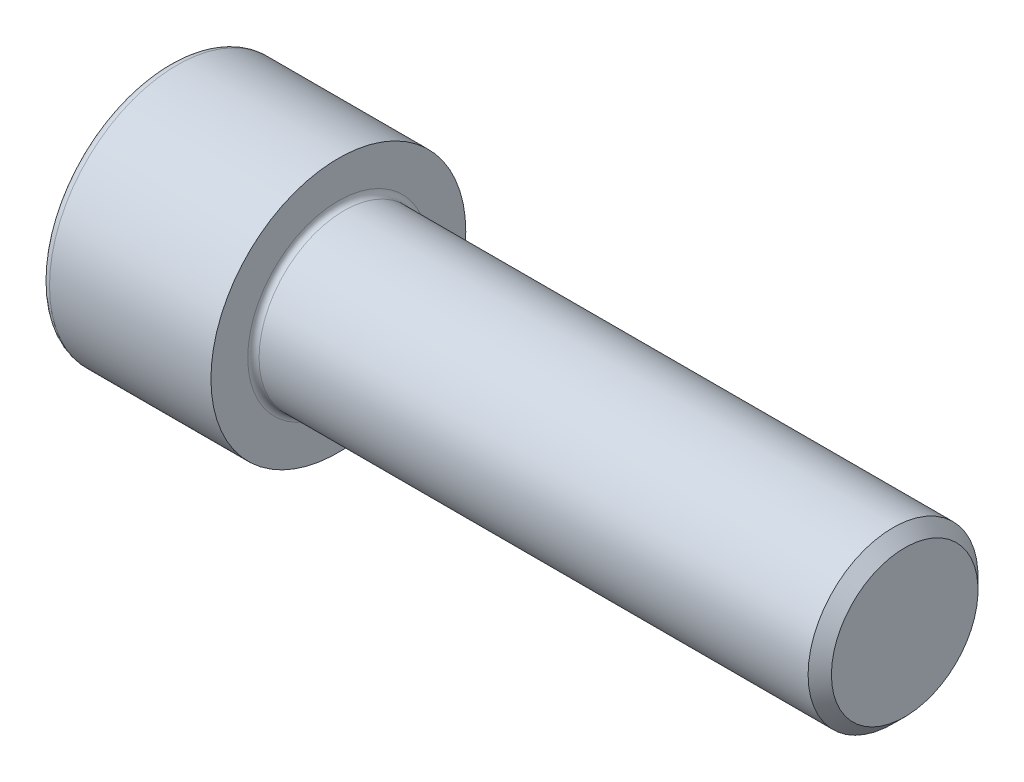
SolidWorks part; units mm, degrees
revolve "Base-Revolve" add sketch "BodySke"
sketch "BodySke" plane through (0, 0, 0) normal (0, 0, 1) x (1, 0, 0)
  line L0 (0, 0) -> (0, 18)
  line L1 (0, 18) -> (24, 18)
  line L2 (24, 18) -> (24, 12)
  line L3 (24, 12) -> (102.352, 12)
  line L4 (104, 10.352) -> (104, 0)
  line L5 (104, 0) -> (0, 0)
  line L6 (-31.75, 0) -> (127, 0) construction
  line L8 (104, 10.352) -> (102.352, 12)
  line L10 (104, -10.352) -> (102.352, -12) construction
  line L11 (27, 9.525) -> (27, 3.175) construction
  line L12 (44, 9.525) -> (44, 3.175) construction
  line L13 (44, 9.525) -> (44, 3.175) construction
cosmetic thread "ThreadCosmetic" [suppressed]
fillet "Fillet1" radius 0.8 1 edges at (24, 0, 12)
fillet "Fillet2" radius 1.2 1 edges at (0, 0, 18)
ref_plane "Plane1" through (0, 0, 0) normal (0, 0, 1) x (1, 0, 0)
ref_plane "Plane2" through (0, 0, 0) normal (0, 1, 0) x (1, 0, 0)
ref_plane "Plane3" through (0, 0, 0) normal (1, 0, 0) x (0, 0, -1)
other "Configuration Table"
sketch "Sketch2" plane through (0, 0, 0) normal (0, 0, 1) x (1, 0, 0)
  line L0 (0, 9.6375) -> (12.573, 9.6375)
  line L1 (12.573, 9.6375) -> (18.1372, 0)
  line L2 (-31.75, 0) -> (127, 0) construction
  line L3 (18.1372, 0) -> (0, 0)
  line L4 (0, 0) -> (0, 9.6375)
  line L6 (0, 0) -> (47.625, 0) construction
revolve "Hex-PreBroach" cut sketch "Sketch2" angle 360 about L6
sketch "Sketch3" plane through (0, 0, 0) normal (-1, 0, 0) x (0, 0.5, 0.866)
  line L0 (5.5642, 9.6375) -> (-5.5642, 9.6375)
  line L1 (-5.5642, 9.6375) -> (-11.1284, 0)
  line L2 (5.5642, 9.6375) -> (11.1284, 0)
  line L3 (5.5642, -9.6375) -> (11.1284, 0)
  line L4 (5.5642, -9.6375) -> (-5.5642, -9.6375)
  line L5 (-5.5642, -9.6375) -> (-11.1284, 0)
extrude "Hex" cut sketch "Sketch3" against normal blind 12.573
sketch "ThdSchSke" plane through (0, 0, 0) normal (0, 0, 1) x (1, 0, 0)
  line L0 (44, -10.352) -> (42.8461, -12)
  line L1 (44, -10.352) -> (45.1539, -12)
  line L2 (45.1539, -12) -> (45.1539, -15)
  line L3 (-3.175, 0) -> (5.1513, 0) construction
  line L4 (0, 16.8) -> (0, -16.8) construction
  line L5 (45.1539, -15) -> (42.8461, -15)
  line L6 (42.8461, -15) -> (42.8461, -12)
revolve "ThreadSchematic" [suppressed] cut sketch "ThdSchSke" angle 360 about L3
pattern_linear "ThdSchPat" [suppressed]
equation "\"D2@Sketch3\" = \"Hex_size@Sketch3\" / 2"
equation "\"D1@Sketch3\" = \"Hex_size@Sketch3\" / 2"
equation "\"D1@Sketch2\" = \"Hex_size@Sketch3\" / 2"
equation "\"Thread_minor@ThreadCosmetic\"  =  \"Minor_dia@BodySke\""
equation "\"Depth@Sketch2\" =  \"Key_eng@Hex\""
equation "\"Thread_length@ThreadCosmetic\" = ((sgn( (\"Length@BodySke\" - \"Advance@BodySke\" * 3.0) - \"Thread_nom@BodySke\" )-1)*( (\"Length@BodySke\" - \"Advance@BodySke\" * 3.0) - \"Thread_nom@BodySke\" ))/-2+ \"Thread_nom@BodySke\""
equation "\"Thread_minor@ThdSchSke\" = \"Minor_dia@BodySke\""
equation "\"Diameter@ThdSchSke\" = \"Diameter@BodySke\""
equation "\"Overcut@ThdSchSke\" = \"Diameter@BodySke\" * 1.25"
equation "\"Start@ThdSchSke\" = \"Head_ht@BodySke\" + \"Length@BodySke\" - \"Thread_length@ThreadCosmetic\"  '---Non-countersunk---"
equation "\"Num_threads@ThdSchPat\" = int( \"Thread_length@ThreadCosmetic\" / \"Advance@BodySke\" + 0.999 )  + 1"
equation "\"Advance@ThdSchPat\" = \"Thread_length@ThreadCosmetic\" /  (\"Num_threads@ThdSchPat\" - 1) 'relax it"
equation "\"Num_threads@ThdSchPat\" = \"Num_threads@ThdSchPat\" - sgn( \"Num_threads@ThdSchPat\" - 1) '---chamfered tips only---"
